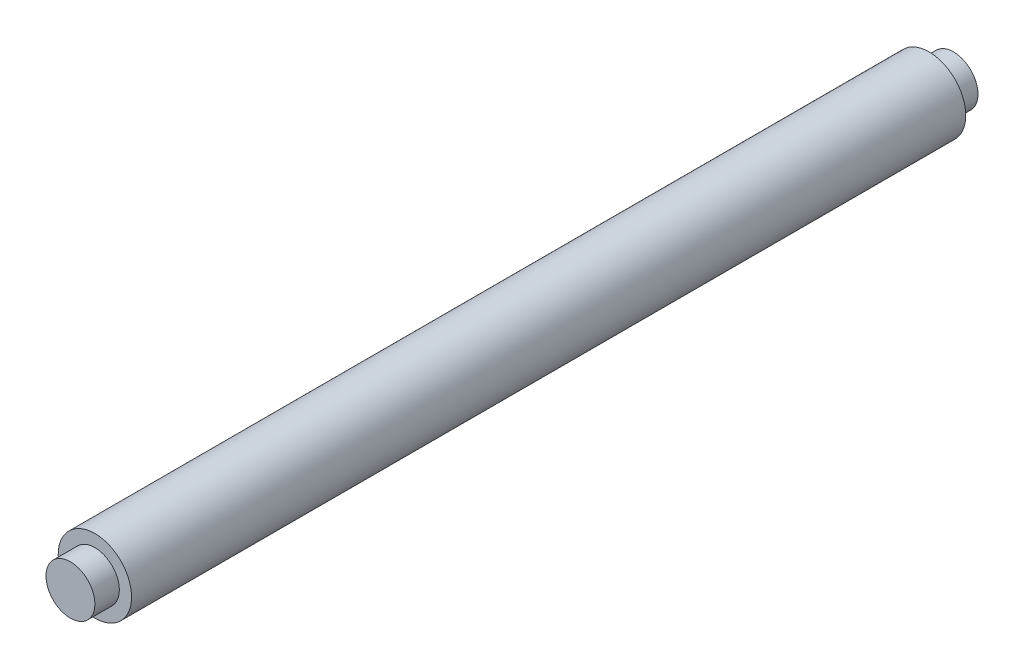
SolidWorks part; units mm, degrees
ref_plane "前视基准面" through (0, 0, 0) normal (0, 0, 1) x (1, 0, 0)
ref_plane "上视基准面" through (0, 0, 0) normal (0, 1, 0) x (1, 0, 0)
ref_plane "右视基准面" through (0, 0, 0) normal (1, 0, 0) x (0, 0, -1)
sketch "草图1" plane through (0, 0, 0) normal (0, 0, 1) x (1, 0, 0)
  circle A0 centre (0, 0) radius 15
  dimension "D1" = 30
extrude "凸台-拉伸1" add sketch "草图1" along normal mid plane 341
sketch "草图2" plane through (0, 0, 170.5) normal (0, 0, 1) x (1, 0, 0)
  circle A0 centre (0, 0) radius 10
  dimension "D1" = 20
extrude "凸台-拉伸2" add sketch "草图2" along normal blind 10
mirror "镜向1" about plane through (0, 0, 0) normal (0, 0, 1) of "凸台-拉伸2"
